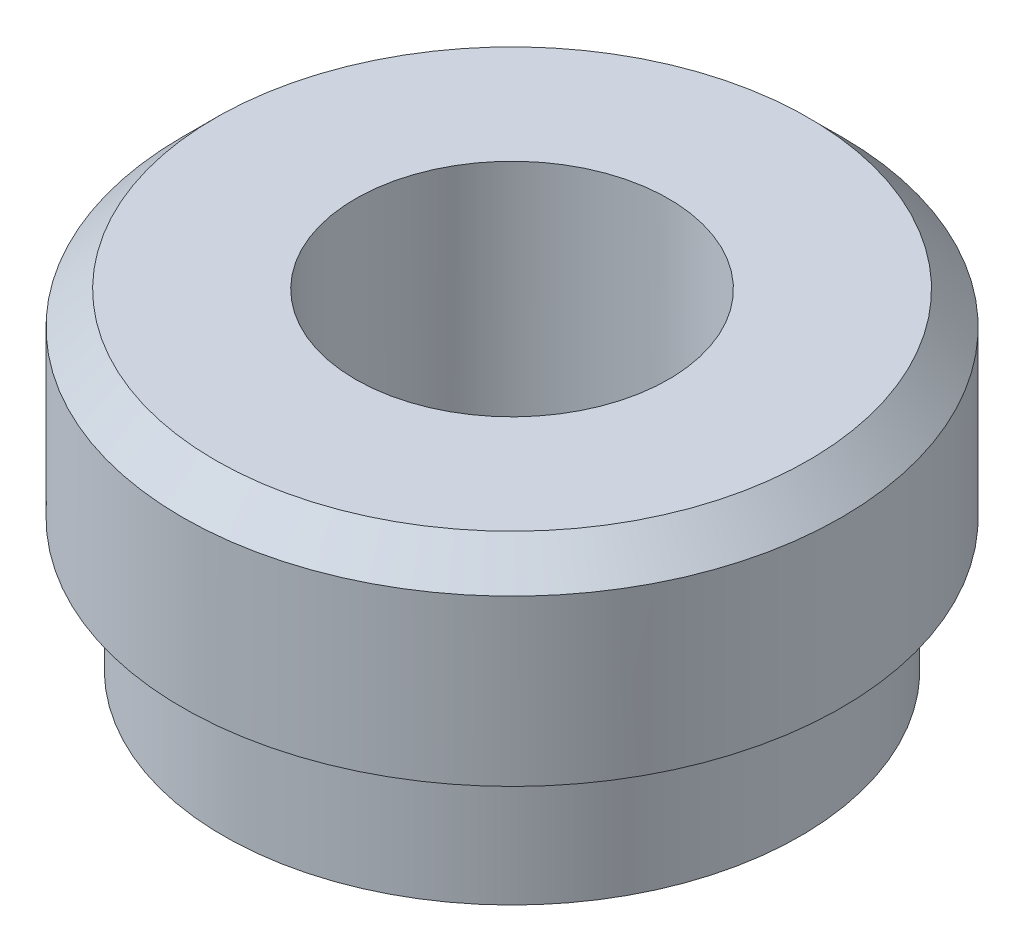
from build123d import *

# Parameters (mm, degrees)
G1_2_TAPPED_HOLE1_D     = 19
G1_2_TAPPED_HOLE1_DEPTH = 47.35
G1_2_TAPPED_HOLE1_TIP   = 5.708175881
CHAMFER1_SIZE           = 2


with BuildPart() as part:
    # Sketch1 → Revolve1 (revolve)
    with BuildSketch(Plane.XY, mode=Mode.PRIVATE) as revolve1_sk:
        Polygon((0, 0), (20, 0), (20, -12), (17.5, -12), (17.5, -20), (0, -20), align=None)
    revolve(revolve1_sk.sketch.rotate(Axis((0, -20, 0), (0, 1, 0)), 90), axis=Axis((0, -20, 0), (0, 1, 0)))

    # G1/2 Tapped Hole1
    with Locations(Plane(origin=(0, 0, 0), x_dir=(1, 0, 0), z_dir=(0, 1, 0))):
        with Locations((0, 0)):
            Hole(G1_2_TAPPED_HOLE1_D / 2, depth=G1_2_TAPPED_HOLE1_DEPTH)
            with Locations((0, 0, -(G1_2_TAPPED_HOLE1_DEPTH + G1_2_TAPPED_HOLE1_TIP / 2))):  # 118° drill point
                Cone(0, G1_2_TAPPED_HOLE1_D / 2, G1_2_TAPPED_HOLE1_TIP, mode=Mode.SUBTRACT)

    # Chamfer1
    chamfer1_edges = [part.edges().sort_by_distance(p)[0] for p in [
        (0, 0, 20),
    ]]
    chamfer(chamfer1_edges, length=CHAMFER1_SIZE)


solid = part.part
